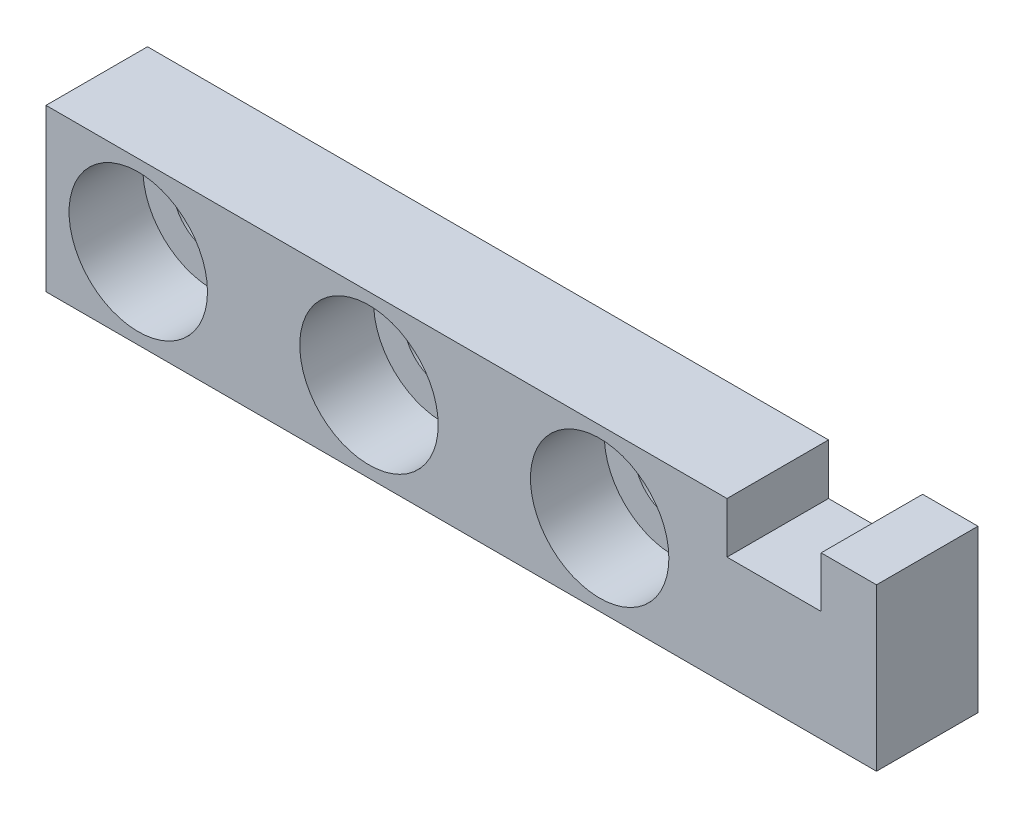
from build123d import *

# Parameters (mm, degrees)
SKETCH1_R           = 4.25
BOSS_EXTRUDE1_DEPTH = 11
SKETCH2_R           = 7.5
CUT_EXTRUDE1_DEPTH  = 8


with BuildPart() as part:
    # Sketch1 → Boss-Extrude1 (new body)
    with BuildSketch(Plane.XY):
        Polygon((-45, 8.75), (28.8, 8.75), (28.8, 3.25), (39, 3.25), (39, 8.75), (45, 8.75), (45, -8.75), (-45, -8.75), align=None)
        with Locations((-35, 0)):
            Circle(SKETCH1_R, mode=Mode.SUBTRACT)
        with Locations((-10, 0)):
            Circle(SKETCH1_R, mode=Mode.SUBTRACT)
        with Locations((15, 0)):
            Circle(SKETCH1_R, mode=Mode.SUBTRACT)
    extrude(amount=BOSS_EXTRUDE1_DEPTH)

    # Sketch2 → Cut-Extrude1 (cut)
    with BuildSketch(Plane.XY.offset(11)):
        with Locations((-35, 0)):
            Circle(SKETCH2_R)
        with Locations((-10, 0)):
            Circle(SKETCH2_R)
        with Locations((15, 0)):
            Circle(SKETCH2_R)
    extrude(amount=-CUT_EXTRUDE1_DEPTH, mode=Mode.SUBTRACT)


solid = part.part
